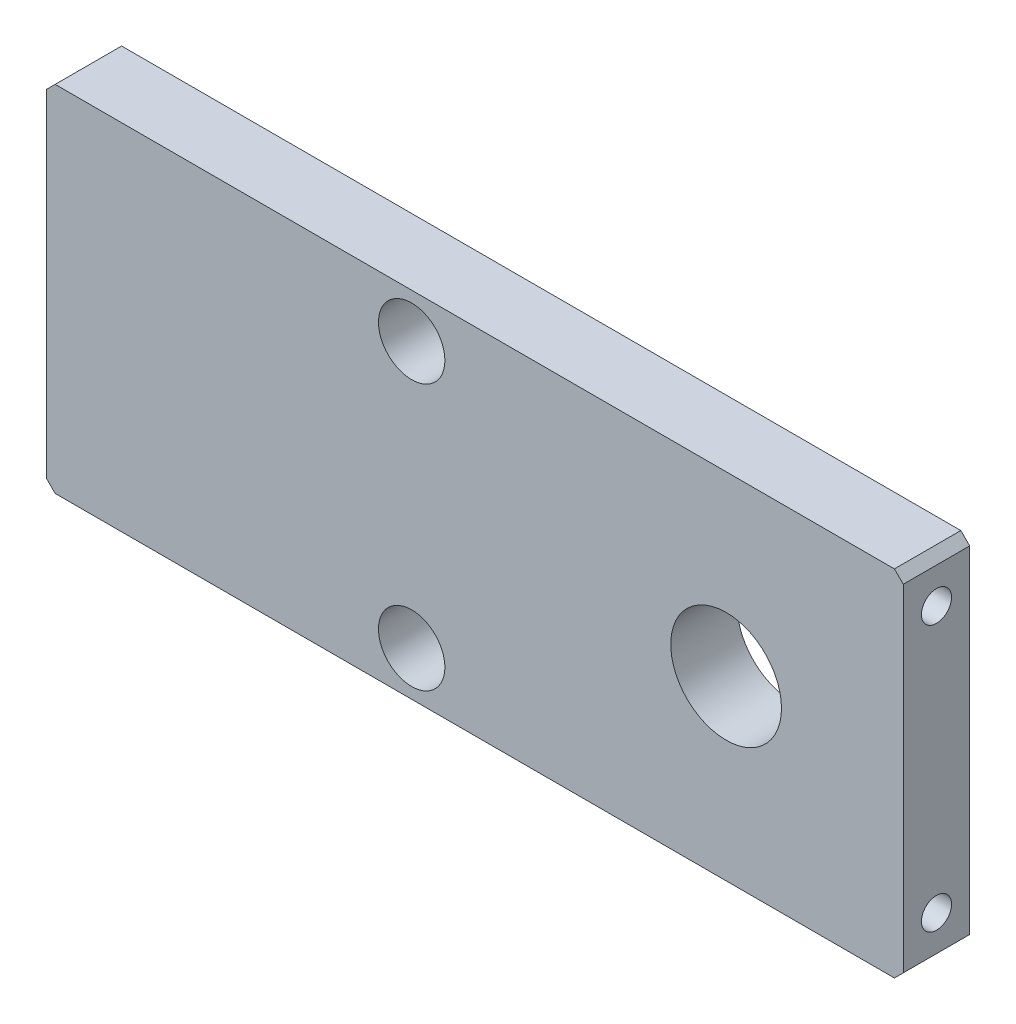
from build123d import *

# Parameters (mm, degrees)
SKETCH_1_W              = 193.5
SKETCH_1_H              = 80
EXTRUDE_1_DEPTH         = 7.5
HOLE_WIZARD_25_0_25_1_D = 25
HOLE_WIZARD_15_0_15_1_D = 15
HOLE_WIZARD_M8_1_D      = 6.8
HOLE_WIZARD_M8_1_DEPTH  = 19.75
HOLE_WIZARD_M8_1_TIP    = 2.042926105
HOLE_WIZARD_M8_2_D      = 6.8
HOLE_WIZARD_M8_2_DEPTH  = 19.75
HOLE_WIZARD_M8_2_TIP    = 2.042926105
SKETCH_11_R             = 56
CUT_EXTRUDE_1_DEPTH     = 10
CHAMFER_1_SIZE          = 2


with BuildPart() as part:
    # 草图1 → 凸台-拉伸1 (new, symmetric)
    with BuildSketch(Plane.XY):
        Rectangle(SKETCH_1_W, SKETCH_1_H)
    extrude(amount=EXTRUDE_1_DEPTH, both=True)

    # Ø25.0 (25) 直径孔1 (through all)
    with Locations(Plane.XY.offset(7.5)):
        with Locations((56.75, 0)):
            Hole(HOLE_WIZARD_25_0_25_1_D / 2)

    # Ø15.0 (15) 直径孔1 (through all)
    with Locations(Plane.XY.offset(7.5)):
        with Locations((-14.25, 30), (-14.25, -30)):
            Hole(HOLE_WIZARD_15_0_15_1_D / 2)

    # M8 螺纹孔1
    with Locations(Plane(origin=(96.75, 0, 0), x_dir=(0, 0, -1), z_dir=(1, 0, 0))):
        with Locations((0, 30), (0, -30)):
            Hole(HOLE_WIZARD_M8_1_D / 2, depth=HOLE_WIZARD_M8_1_DEPTH)
            with Locations((0, 0, -(HOLE_WIZARD_M8_1_DEPTH + HOLE_WIZARD_M8_1_TIP / 2))):  # 118° drill point
                Cone(0, HOLE_WIZARD_M8_1_D / 2, HOLE_WIZARD_M8_1_TIP, mode=Mode.SUBTRACT)

    # M8 螺纹孔2
    with Locations(Plane.ZY.offset(96.75)):
        with Locations((0, 30), (0, -30)):
            Hole(HOLE_WIZARD_M8_2_D / 2, depth=HOLE_WIZARD_M8_2_DEPTH)
            with Locations((0, 0, -(HOLE_WIZARD_M8_2_DEPTH + HOLE_WIZARD_M8_2_TIP / 2))):  # 118° drill point
                Cone(0, HOLE_WIZARD_M8_2_D / 2, HOLE_WIZARD_M8_2_TIP, mode=Mode.SUBTRACT)

    # 草图11 → 切除-拉伸1 (cut)
    with BuildSketch(Plane.ZY.offset(96.75)):
        with Locations((-52.5, 0)):
            Circle(SKETCH_11_R)
    extrude(amount=-CUT_EXTRUDE_1_DEPTH, mode=Mode.SUBTRACT)

    # 倒角1
    chamfer_1_edges = [part.edges().sort_by_distance(p)[0] for p in [
        (96.75, -40, 0),
        (-96.75, -40, 0),
        (-96.75, 40, 0),
        (96.75, 40, 0),
    ]]
    chamfer(chamfer_1_edges, length=CHAMFER_1_SIZE)


solid = part.part
